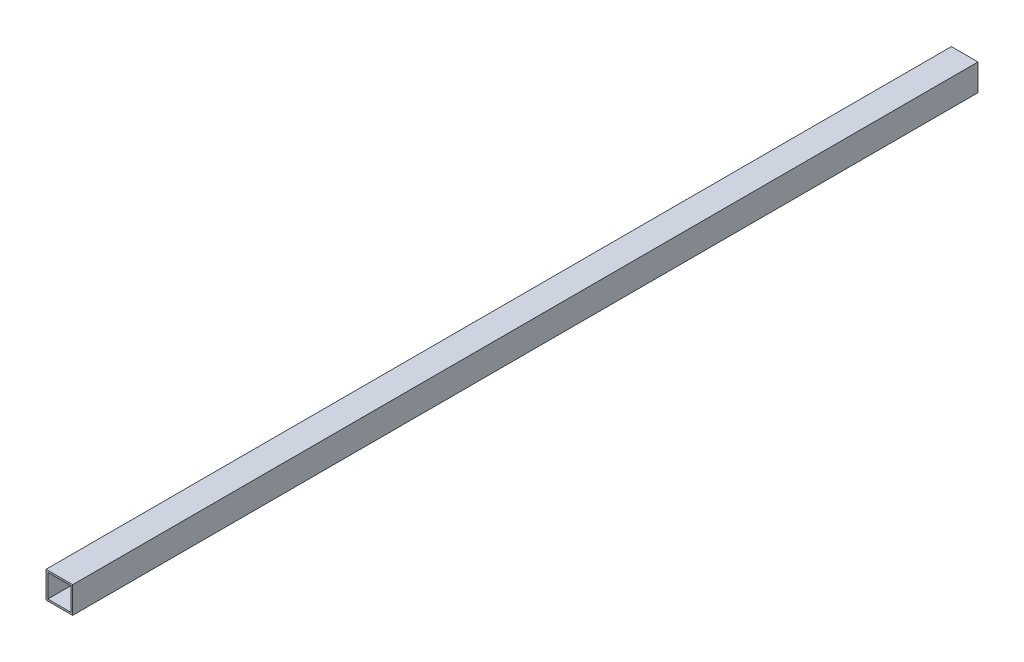
from build123d import *

# Parameters (mm, degrees)
SKETCH_1_W      = 30
SKETCH_1_H      = 30
SKETCH_1_W_2    = 26
SKETCH_1_H_2    = 26
EXTRUDE_1_DEPTH = 510


with BuildPart() as part:
    # 草图1 → 凸台-拉伸1 (new, symmetric)
    with BuildSketch(Plane.XY):
        Rectangle(SKETCH_1_W, SKETCH_1_H)
        Rectangle(SKETCH_1_W_2, SKETCH_1_H_2, mode=Mode.SUBTRACT)
    extrude(amount=EXTRUDE_1_DEPTH, both=True)


solid = part.part
